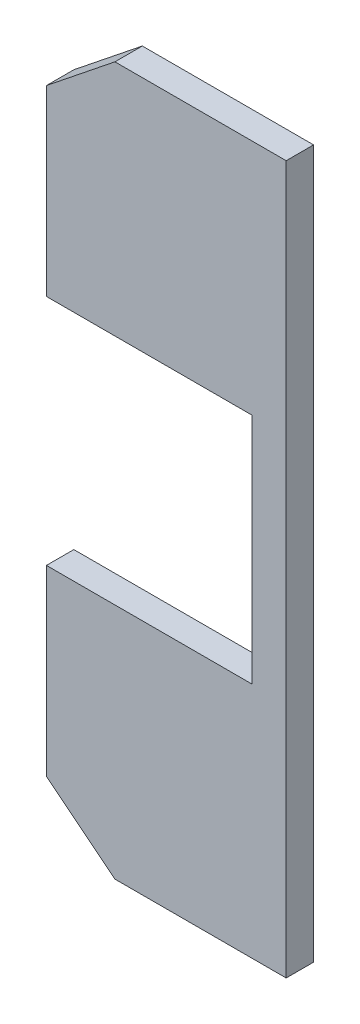
from build123d import *

# Parameters (mm, degrees)
SKETCH1_W      = 15
SKETCH1_H      = 310
EXTRUDE1_DEPTH = 6
EXTRUDE3_DEPTH = 6


with BuildPart() as part:
    # Sketch1 → Extrude1 (new, symmetric)
    with BuildSketch(Plane.XY):
        Rectangle(SKETCH1_W, SKETCH1_H)
    extrude(amount=EXTRUDE1_DEPTH, both=True)

    # Sketch3 → Extrude3 (add, symmetric)
    with BuildSketch(Plane.XY):
        Polygon((-7.5, 155), (-67.5, 155), (-97.5, 131), (-97.5, 51), (-7.5, 51), align=None)
        Polygon((-7.5, -51), (-7.5, -155), (-67.5, -155), (-97.5, -131), (-97.5, -51), align=None)
    extrude(amount=EXTRUDE3_DEPTH, both=True)


solid = part.part
